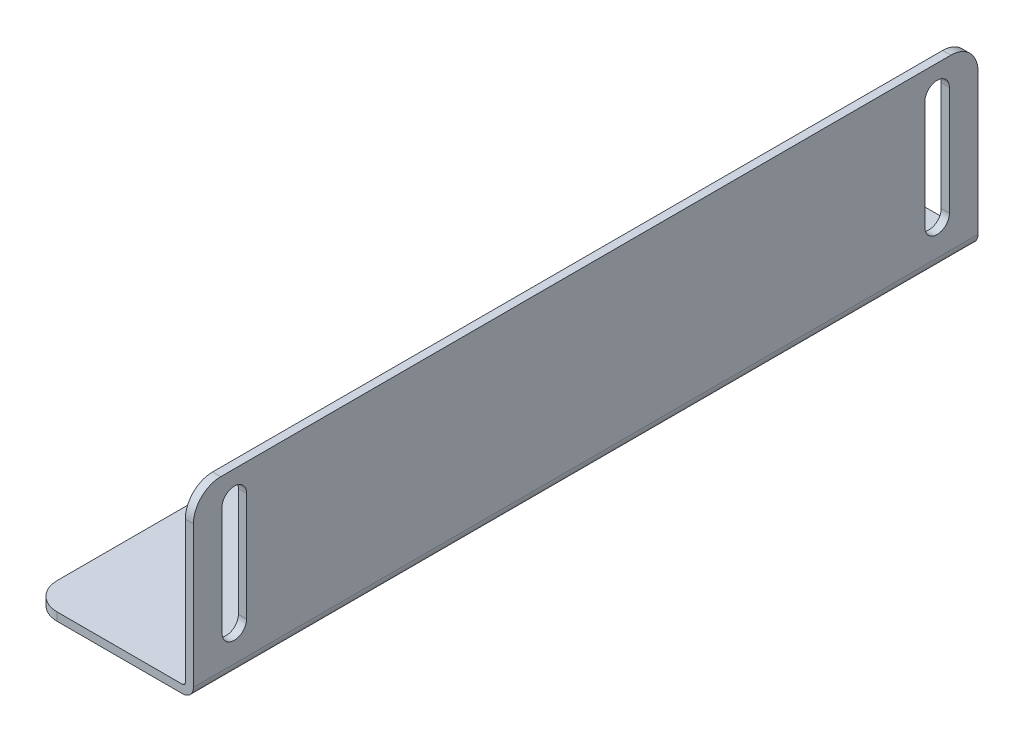
from build123d import *

# Parameters (mm, degrees)
SKETCH_1_W          = 30
SKETCH_1_H          = 33
EXTRUDE_1_DEPTH     = 144
SHELL_1_T           = -1.5
FILLET_1_R          = 5
FILLET_2_R          = 0.5
FILLET_3_R          = 2
CUT_EXTRUDE_1_DEPTH = 198.864221121
CUT_EXTRUDE_2_REACH = 152.748
SKETCH_3_R          = 1.75
CUT_EXTRUDE_3_DEPTH = 1.5


with BuildPart() as part:
    # 草图1 → 凸台-拉伸1 (new body)
    with BuildSketch(Plane.XY):
        with Locations((15, 16.5)):
            Rectangle(SKETCH_1_W, SKETCH_1_H)
    extrude(amount=EXTRUDE_1_DEPTH)

    # 抽壳1
    shell_1_openings = [part.faces().sort_by_distance(p)[0] for p in [
        (15, 16.5, 144),
        (15, 16.5, 0),
        (15, 33, 72),
        (0, 16.5, 72),
    ]]
    offset(amount=SHELL_1_T, openings=shell_1_openings, kind=Kind.INTERSECTION)

    # 圆角1
    fillet_1_edges = [part.edges().sort_by_distance(p)[0] for p in [
        (29.25, 33, 144),
        (0, 0.75, 144),
        (29.25, 33, 0),
        (0, 0.75, 0),
    ]]
    fillet(fillet_1_edges, radius=FILLET_1_R)

    # 圆角2
    fillet_2_edges = [part.edges().sort_by_distance(p)[0] for p in [
        (28.5, 1.5, 72),
    ]]
    fillet(fillet_2_edges, radius=FILLET_2_R)

    # 圆角3
    fillet_3_edges = [part.edges().sort_by_distance(p)[0] for p in [
        (30, 0, 72),
    ]]
    fillet(fillet_3_edges, radius=FILLET_3_R)

    # 草图2 → 切除-拉伸1 (cut, through all)
    with BuildSketch(Plane(origin=(28.5, 0, -49), x_dir=(0, 0, 1), z_dir=(-1, 0, 0))):
        with BuildLine():
            Line((54.25, 8), (54.25, 28))
            ThreePointArc((54.25, 28), (56.5, 30.25), (58.75, 28))
            Line((58.75, 28), (58.75, 8))
            ThreePointArc((58.75, 8), (56.5, 5.75), (54.25, 8))
        make_face()
        with BuildLine():
            Line((187.75, 28), (187.75, 8))
            ThreePointArc((187.75, 8), (185.5, 5.75), (183.25, 8))
            Line((183.25, 8), (183.25, 28))
            ThreePointArc((183.25, 28), (185.5, 30.25), (187.75, 28))
        make_face()
    extrude(amount=-CUT_EXTRUDE_1_DEPTH, mode=Mode.SUBTRACT)

    # 草图3 → 切除-拉伸2 (cut, up to next)
    with BuildSketch(Plane(origin=(0, 0, 0), x_dir=(1, 0, 0), z_dir=(0, 1, 0)), mode=Mode.PRIVATE) as cut_extrude_2_sk1:
        with Locations(Location((5, -87.875, 0), (0, 0, 270))):
            Circle(SKETCH_3_R)
    cut_extrude_2_tool1 = extrude(cut_extrude_2_sk1.sketch, amount=CUT_EXTRUDE_2_REACH, mode=Mode.PRIVATE) & part.part
    # 草图3 → 切除-拉伸2 (cut, up to next)
    with BuildSketch(Plane(origin=(0, 0, 0), x_dir=(1, 0, 0), z_dir=(0, 1, 0)), mode=Mode.PRIVATE) as cut_extrude_2_sk2:
        with Locations(Location((5, -56.125, 0), (0, 0, 270))):
            Circle(SKETCH_3_R)
    cut_extrude_2_tool2 = extrude(cut_extrude_2_sk2.sketch, amount=CUT_EXTRUDE_2_REACH, mode=Mode.PRIVATE) & part.part
    add(cut_extrude_2_tool1.solids().sort_by_distance((5, 0, 87.875))[0], mode=Mode.SUBTRACT)
    add(cut_extrude_2_tool2.solids().sort_by_distance((5, 0, 56.125))[0], mode=Mode.SUBTRACT)

    # 草图4 → 切除-拉伸3 (cut)
    with BuildSketch(Plane(origin=(0, 0, 0), x_dir=(1, 0, 0), z_dir=(0, 1, 0))):
        with BuildLine():
            Line((3.25, -100.375), (3.25, -75.375))
            ThreePointArc((3.25, -75.375), (5, -73.625), (6.75, -75.375))
            Line((6.75, -75.375), (6.75, -100.375))
            ThreePointArc((6.75, -100.375), (5, -102.125), (3.25, -100.375))
        make_face()
        with BuildLine():
            Line((3.25, -68.625), (3.25, -43.625))
            ThreePointArc((3.25, -43.625), (5, -41.875), (6.75, -43.625))
            Line((6.75, -43.625), (6.75, -68.625))
            ThreePointArc((6.75, -68.625), (5, -70.375), (3.25, -68.625))
        make_face()
    extrude(amount=CUT_EXTRUDE_3_DEPTH, mode=Mode.SUBTRACT)


solid = part.part
